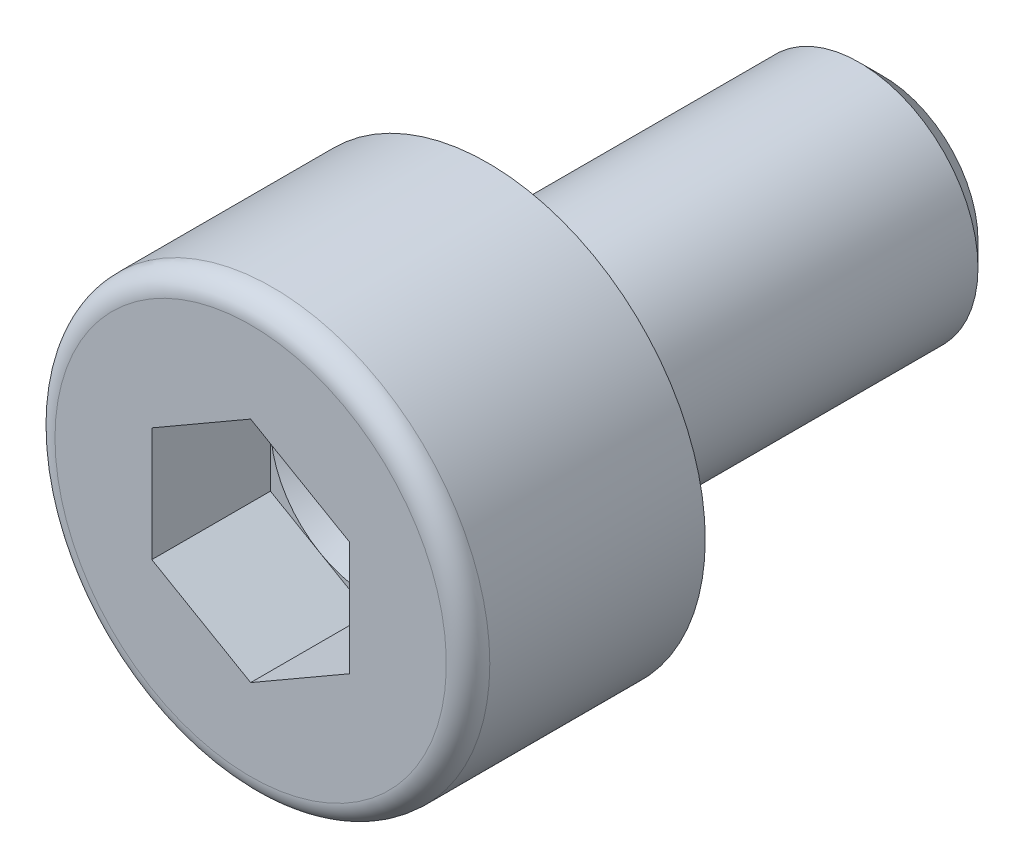
from build123d import *

# Parameters (mm, degrees)
CUT_EXTRUDE1_DEPTH = 1.5
FILLET1_R          = 0.275
CHAMFER1_SIZE      = 0.3
FILLET2_R          = 0.125


with BuildPart() as part:
    # Sketch3 → Revolve1 (revolve)
    with BuildSketch(Plane(origin=(0, 0, 0), x_dir=(0, 0, -1), z_dir=(1, 0, 0)), mode=Mode.PRIVATE) as revolve1_sk:
        Polygon((-3, 0.6), (-3, 2.75), (0, 2.75), (0, 1.5), (5, 1.5), (5, 0.6), align=None)
    revolve(revolve1_sk.sketch.rotate(Axis((0, 0, 3), (0, 0, -1)), 90), axis=Axis((0, 0, 3), (0, 0, -1)))

    # Sketch4 → Cut-Extrude1 (cut)
    with BuildSketch(Plane.XY.offset(3)):
        Polygon((0, 1.443375673), (-1.25, 0.721687836), (-1.25, -0.721687836), (0, -1.443375673), (1.25, -0.721687836), (1.25, 0.721687836), align=None)
    extrude(amount=-CUT_EXTRUDE1_DEPTH, mode=Mode.SUBTRACT)

    # Fillet1
    fillet1_edges = [part.edges().sort_by_distance(p)[0] for p in [
        (-2.75, 0, 3),
    ]]
    fillet(fillet1_edges, radius=FILLET1_R)

    # Chamfer1
    chamfer1_edges = [part.edges().sort_by_distance(p)[0] for p in [
        (-1.5, 0, -5),
    ]]
    chamfer(chamfer1_edges, length=CHAMFER1_SIZE)

    # Cut-Extrude2 cone 1 section (through the dimple's axis) → Cut-Extrude2 (revolve, cut)
    with BuildSketch(Plane(origin=(0, 0, 1.5), x_dir=(0, -1, 0), z_dir=(1, 0, 0))):
        Polygon((0, 0), (1.25, 0), (0, 0.721687836), align=None)
    revolve(axis=Axis((0, 0, 1.5), (0, 0, -1)), mode=Mode.SUBTRACT)

    # Fillet2
    fillet2_edges = [part.edges().sort_by_distance(p)[0] for p in [
        (-1.5, 0, 0),
    ]]
    fillet(fillet2_edges, radius=FILLET2_R)


solid = part.part
